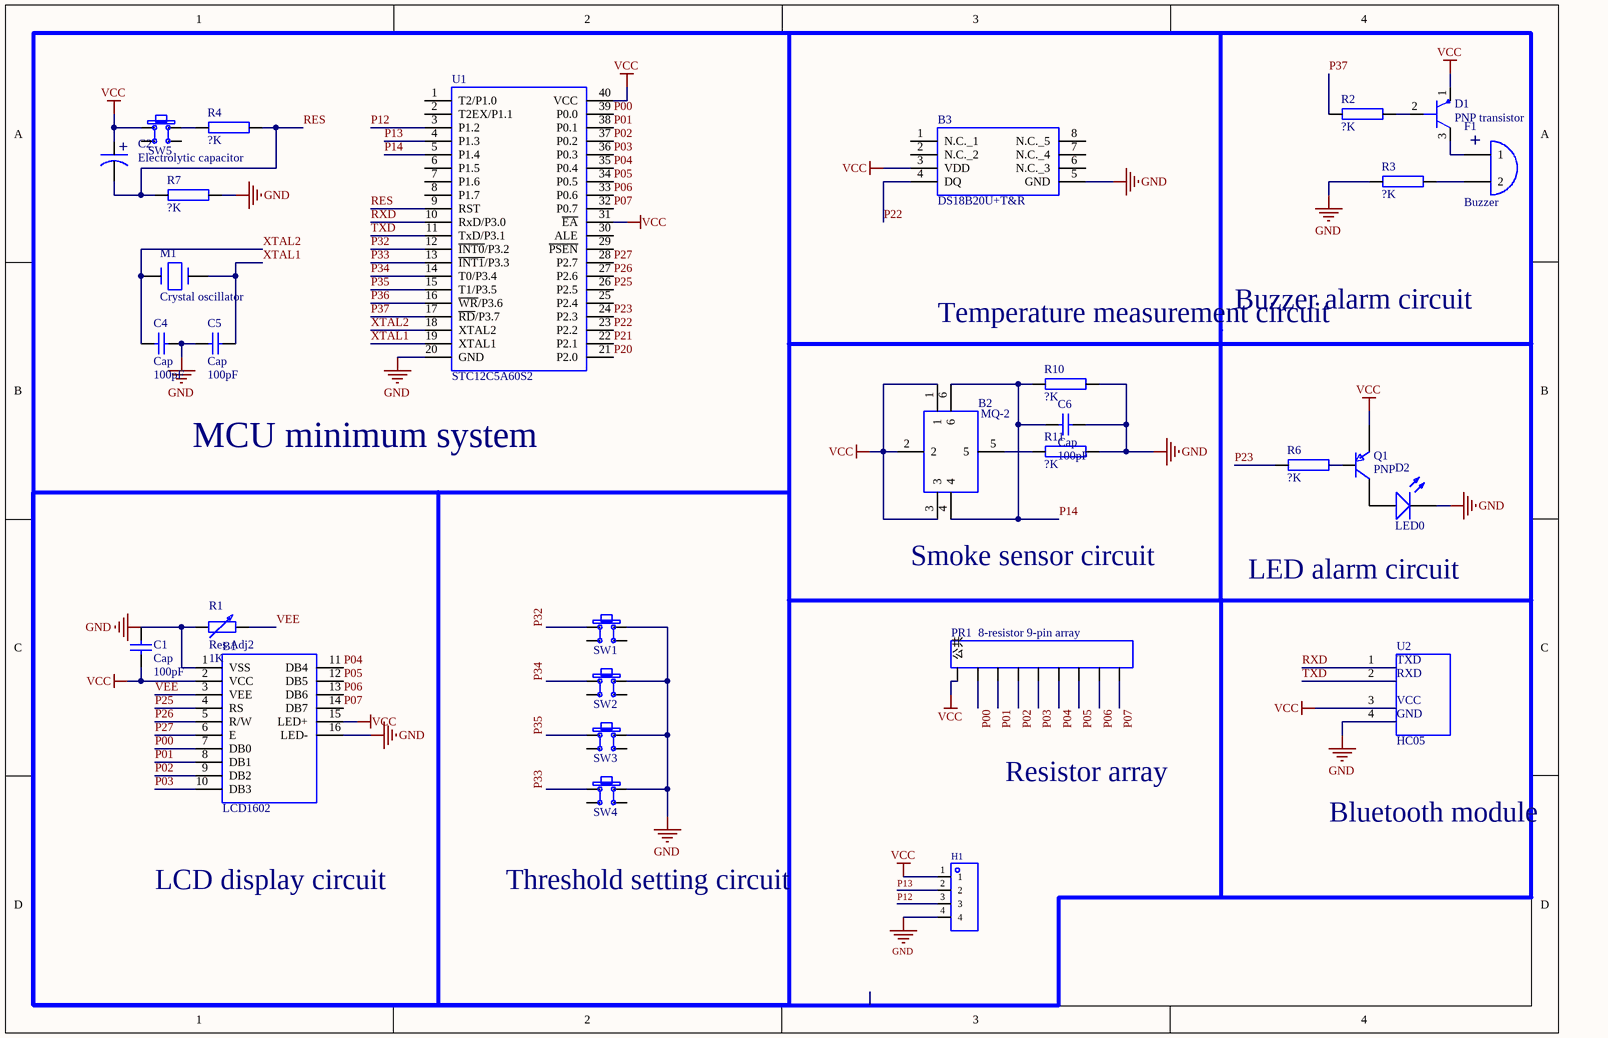
[diagram p0: MISC75421-3.schdoc]
# Altium project MISC75421-2.PrjPcb
1 sheet, 30 parts. Net scope: global (net labels, ports and power ports of the same name join across sheets).
Board file: MISC75421.pcbdoc

## Sheet MISC75421-3.schdoc
size 292 x 193 mm; Name: MISC75421

### Parts
B1  LCD1602  [LCD1602]
B2  MQ-2  [SENSOR-TH_MQ-2]
B3  DS18B20U+T&R  [HDR-TH_8P-P2.54-V-F-R2-C4-S2.54-1]
C1  Cap  value 100pF  [RAD-0.3]
C2  Electrolytic capacitor  [CAP-TH_BD5.0-P2.00-D0.8-FD-10UF50VC110GL]
C4  Cap  value 100pF  [RAD-0.3]
C5  Cap  value 100pF  [RAD-0.3]
C6  Cap  value 100pF  [RAD-0.3]
D1  PNP transistor  [S8550P_TO-92]
D2  LED0  [LED-TH_5mm]
F1  Buzzer  [BUZ-TH_BD12.0-P6.00-D0.9-RD]
H1  (no value)  [HDR-TH_4P-P2.54-V-F]
M1  Crystal oscillator  [HC-49S_L11.5-W5.0-P4.88]
PR1  8-resistor 9-pin array  [RES-ARRAY-TH_9P-P2.54-D1.0]
Q1  PNP  [TO-92-3_L4.6-W3.6-P1.27-L_1]
R1  Res Adj2  value 1K  [RES-ADJ-TH_3P-L9.5-W4.85-P2.54_PV36W103C01B00]
R2  ?K  [Res_1/4W]
R3  ?K  [Res_1/4W]
R4  ?K  [Res_1/4W]
R6  ?K  [Res_1/4W]
R7  ?K  [Res_1/4W]
R10  ?K  [Res_1/4W]
R11  ?K  [Res_1/4W]
SW1  TSW tactile switch  [SW-TH_4P-L6.0-W6.0-P4.50-LS6.5]  (value not drawn)
SW2  TSW tactile switch  [SW-TH_4P-L6.0-W6.0-P4.50-LS6.5]  (value not drawn)
SW3  TSW tactile switch  [SW-TH_4P-L6.0-W6.0-P4.50-LS6.5]  (value not drawn)
SW4  TSW tactile switch  [SW-TH_4P-L6.0-W6.0-P4.50-LS6.5]  (value not drawn)
SW5  TSW tactile switch  [SW-TH_4P-L6.0-W6.0-P4.50-LS6.5]  (value not drawn)
U1  STC12C5A60S2  [DIP-40_L52.3-W13.9-P2.54-LS15.2-BL-BASE]
U2  HC05  [HDR-TH_4P-P2.54-V-F]

### Nets
GND: B1.1(VSS) B1.16(LED-) B3.5(GND) C1.2 C4.2 C5.1 C6.1 D2.2(K) H1.4 R1.1 R3.2 R7.2 R10.2 R11.2 SW1.4 SW2.4 SW3.4 SW4.4 U1.20(GND) U2.4(GND)
VCC: B1.2(VCC) B1.15(LED+) B2.1 B2.2 B2.3 B3.3(VDD) C1.1 C2.1 D1.1(E) H1.1 PR1.1(公共) Q1.3(E) SW5.1 U1.31(~{EA}) U1.40(VCC) U2.3(VCC)
P00: B1.7(DB0) PR1.2 U1.39(P0.0)
P01: B1.8(DB1) PR1.3 U1.38(P0.1)
P02: B1.9(DB2) PR1.4 U1.37(P0.2)
P03: B1.10(DB3) PR1.5 U1.36(P0.3)
P04: B1.11(DB4) PR1.6 U1.35(P0.4)
P05: B1.12(DB5) PR1.7 U1.34(P0.5)
P06: B1.13(DB6) PR1.8 U1.33(P0.6)
P07: B1.14(DB7) PR1.9 U1.32(P0.7)
P12: H1.3 U1.3(P1.2)
P13: H1.2 U1.4(P1.3)
P14: B2.4 B2.6 C6.2 R10.1 U1.5(P1.4)
P20: U1.21(P2.0)
P21: U1.22(P2.1)
P22: B3.4(DQ) U1.23(P2.2)
P23: R6.1 U1.24(P2.3)
P25: B1.4(RS) U1.26(P2.5)
P26: B1.5(R/W) U1.27(P2.6)
P27: B1.6(E) U1.28(P2.7)
P32: SW1.1 U1.12(~{INT0}/P3.2)
P33: SW4.1 U1.13(~{INT1}/P3.3)
P34: SW2.1 U1.14(T0/P3.4)
P35: SW3.1 U1.15(T1/P3.5)
P36: U1.16(~{WR}/P3.6)
P37: R2.1 U1.17(~{RD}/P3.7)
RES: C2.2 R4.2 R7.1 U1.9(RST)
RXD: U1.10(RxD/P3.0) U2.1(TXD)
TXD: U1.11(TxD/P3.1) U2.2(RXD)
VEE: B1.3(VEE) R1.2
XTAL1: C5.2 M1.2 U1.19(XTAL1)
XTAL2: C4.1 M1.1 U1.18(XTAL2)
NetB2_5: B2.5 R11.1
NetD1_2: D1.2(B) R2.2
NetD1_3: D1.3(C) F1.1
NetD2_1: D2.1(A) Q1.1(C)
NetF1_2: F1.2 R3.1
NetQ1_2: Q1.2(B) R6.2
NetR4_1: R4.1 SW5.4

Not connected (* = marked no-connect by the designer): B3 1(N.C._1) 2(N.C._2) 6(N.C._3) 7(N.C._4) 8(N.C._5); SW1 2 3; SW2 2 3; SW3 2 3; SW4 2 3; SW5 2 3; U1 1(T2/P1.0) 2(T2EX/P1.1) 6(P1.5) 7(P1.6) 8(P1.7) 25(P2.4) 29(~{PSEN}) 30(ALE)

### Notes on the sheet
- Buzzer alarm circuit
- Temperature measurement circuit
- MCU minimum system
- (near B2) Smoke sensor circuit
- LED alarm circuit
- Resistor array
- Bluetooth module
- LCD display circuit
- Threshold setting circuit

### Library data of the parts
B1 = LCD1602: Character LCD Module 1602 Built in Controller St7066u COB Type LCD; Manufacturer_Name: Waveshare; Geometry.Height: 14mm; UniqueId: ecd4cc2f475f8764; AddInBom: yes; ModelId: f9d832f46a914cadb50fc4d4cefd2517; Device: LCD1602; Manufacturer_Part_Number: LCD1602; Mouser Part Number: *; Mouser Price/Stock: *; Arrow Part Number: *; Arrow Price/Stock: *; Datasheet Link: https://www.waveshare.com/datasheet/LCD_en_PDF/LCD1602.pdf; DesignItemID: LCD1602; LibraryName: LCD1602; SymbolName: LCD1602; FootprintName: LCD1602; ModelName: LCD1602; ConvertToPcb: yes
B2 = MQ-2: Sensor: gas; smoke,combustible gases; Range: 30010000ppm; MQ-2; Manufacturer_Name: WINSEN; Geometry.Height: 15mm; Origin Footprint: MQ2; UniqueId: 09c8abc5601f23af; AddInBom: yes; Device: MQ-2; Manufacturer_Part_Number: MQ-2; Mouser Part Number: *; Mouser Price/Stock: *; Arrow Part Number: *; Arrow Price/Stock: *; Datasheet Link: https://www.tme.com/Document/9f6250807cbcd9cc73a92775a9c66d2e/MQ-2.pdf; DesignItemID: MQ-2; LibraryName: MQ-2; SymbolName: MQ-2
B3 = DS18B20U+T&R: Board Mount Temperature Sensors Prgmble Resolution 1-Wire Parasite Pwr; Manufacturer_Name: Analog Devices; Geometry.Height: 1.1mm; Origin Footprint: SOP65P490X110-8N; UniqueId: 602cac6f5ce6261d; AddInBom: yes; Device: DS18B20U+T&R; Manufacturer_Part_Number: DS18B20U+T&R; Mouser Part Number: 700-DS18B20UT&R; Mouser Price/Stock: https://www.mouser.co.uk/ProductDetail/Analog-Devices-Maxim-Integrated/DS18B20U%2bTR?qs=7H2Jq%252ByxpJI1ACKb6RIQLA%3D%3D; Arrow Part Number: DS18B20U+T&R; Arrow Price/Stock: https://www.arrow.com/en/products/ds18b20utr/analog-devices?utm_currency=USD&region=nac; Datasheet Link: https://datasheets.maximintegrated.com/en/ds/DS18B20.pdf; DesignItemID: DS18B20U+T&R; LibraryName: DS18B20U+T&R; SymbolName: DS18B20U+T&R
C1 = Cap: Capacitor; UniqueId: 5fb4f22ffcb6a001; AddInBom: yes; Device: Cap; Published: 8-Jun-2000; LatestRevisionDate: 17-Jul-2002; LatestRevisionNote: Re-released for DXP Platform.; PackageReference: RAD-0.3; PackageDescription: Radial Cap, Thru-Hole; 2 Leads; 0.3 in Pin Spacing; DesignItemID: Cap; LibraryName: Miscellaneous Devices; SymbolName: Cap; FootprintName: RAD-0.3; Publisher: Altium Limited
C2 = 电解电容: Origin Footprint: 电解电容-2.5mm; OriginFootprint 2: 电解电容-5mm; UniqueId: 21d50210554cb61f; AddInBom: yes; Device: Electrolytic capacitor; DesignItemID: 电解电容; LibraryName: Common component library; SymbolName: Electrolytic capacitor
C4 = Cap: Capacitor; UniqueId: 623e2bb2442f04df; AddInBom: yes; Device: Cap; Published: 8-Jun-2000; LatestRevisionDate: 17-Jul-2002; LatestRevisionNote: Re-released for DXP Platform.; PackageReference: RAD-0.3; PackageDescription: Radial Cap, Thru-Hole; 2 Leads; 0.3 in Pin Spacing; DesignItemID: Cap; LibraryName: Miscellaneous Devices; SymbolName: Cap; FootprintName: RAD-0.3; Publisher: Altium Limited
C5 = Cap: Capacitor; UniqueId: 05d417a4d81547fc; AddInBom: yes; Device: Cap; Published: 8-Jun-2000; LatestRevisionDate: 17-Jul-2002; LatestRevisionNote: Re-released for DXP Platform.; PackageReference: RAD-0.3; PackageDescription: Radial Cap, Thru-Hole; 2 Leads; 0.3 in Pin Spacing; DesignItemID: Cap; LibraryName: Miscellaneous Devices; SymbolName: Cap; FootprintName: RAD-0.3; Publisher: Altium Limited
C6 = Cap: Capacitor; UniqueId: d45ffe04e43665a4; AddInBom: yes; Device: Cap; Published: 8-Jun-2000; LatestRevisionDate: 17-Jul-2002; LatestRevisionNote: Re-released for DXP Platform.; PackageReference: RAD-0.3; PackageDescription: Radial Cap, Thru-Hole; 2 Leads; 0.3 in Pin Spacing; DesignItemID: Cap; LibraryName: Miscellaneous Devices; SymbolName: Cap; FootprintName: RAD-0.3; Publisher: Altium Limited
D1 = PNP三极管: UniqueId: 07a0d5848cd81316; AddInBom: yes; Device: PNP transistor; Origin Footprint: Transistor; DesignItemID: PNP三极管; LibraryName: Dedicated component library; SymbolName: PNP transistor; ConvertToPcb: yes
D2 = LED0: Typical INFRARED GaAs LED; Origin Footprint: LED-0; UniqueId: fa5cd661465da5bc; AddInBom: yes; Device: LED0; Published: 8-Jun-2000; LatestRevisionDate: 08-Jul-2005; LatestRevisionNote: Mech Layer 1 removed.; PackageReference: LED-0; PackageDescription: LED; 2 Leads; DesignItemID: LED0; LibraryName: Miscellaneous Devices; SymbolName: LED0; Publisher: Altium Limited
F1 = 蜂鸣器: UniqueId: 0327748d3d32b991; AddInBom: yes; Device: Buzzer; Origin Footprint: Buzzer; DesignItemID: 蜂鸣器; LibraryName: Dedicated component library; SymbolName: Buzzer
H1 = HDR-F_2.54_1x4P: Symbol: 2.54-1*4P female; ConvertToPcb: yes; ModelId: d187812051054f85879fcaa51a310d8e0819f05c4eef4c71ace90d822a990e87; ModelTransform: 419.6842,98.464,0,0,0,0,0,0,-118.11; Device: HDR-F_2.54_1x4P; AddInBom: yes; SupplierPart: C2718488; Supplier Footprint: 插件; FootprintName: HDR-TH_4P-P2.54-V-F; ModelName: HDR-TH_4P-P2.54-V-F
M1 = 晶振: UniqueId: dd3285c2b6d2a98e; AddInBom: yes; Device: Crystal oscillator; Origin Footprint: Crystal oscillator; DesignItemID: 晶振; LibraryName: Common component library; SymbolName: Crystal oscillator
PR1 = 8阻9排: UniqueId: d5ea52400f8981b9; AddInBom: yes; Device: 8-resistor 9-pin array; Origin Footprint: 8-resistor 9-pin array; DesignItemID: 8阻9排; LibraryName: Common component library; SymbolName: 8-resistor 9-pin array
Q1 = PNP: PNP Bipolar Transistor; Origin Footprint: SOT-23B_N; OriginFootprint 2: SOT-23B_M; UniqueId: 047b734180970fea; AddInBom: yes; Device: PNP; Published: 8-Jun-2000; LatestRevisionDate: 29-May-2009; LatestRevisionNote: IPC-7351 Footprint Added.; PackageVersion: Aug-1999; PackageReference: SOT-23B; PackageDescription: 3-Pin SOT-23 Package 0.95 mm Pitch, 2.4 mm Lead Span; DesignItemID: PNP; LibraryName: Miscellaneous Devices; SymbolName: PNP; Publisher: Altium Limited
R1 = Res Adj2: Variable Resistor; Set Position: 0.5; Origin Footprint: AXIAL-0.6; UniqueId: 4e166b190d4de1c3; AddInBom: yes; Device: Res Adj2; Published: 8-Jun-2000; LatestRevisionDate: 17-Jul-2002; LatestRevisionNote: Re-released for DXP Platform.; PackageReference: AXIAL-0.6; PackageDescription: Axial Device, Thru-Hole; 2 Leads; 0.6 in Pin Spacing; DesignItemID: Res Adj2; LibraryName: Miscellaneous Devices; SymbolName: Res Adj2; Publisher: Altium Limited
R2 = ？K: Origin Footprint: R general resistor/10mm; UniqueId: 06442d24ab060343; SymbolName: R general resistor; AddInBom: yes; Device: ?K; DesignItemID: R一般电阻; LibraryName: Dedicated component library
R3 = ？K: Origin Footprint: R general resistor/10mm; UniqueId: 6e26aea592918673; SymbolName: R general resistor; AddInBom: yes; Device: ?K; DesignItemID: R一般电阻; LibraryName: Dedicated component library
R4 = ？K: Origin Footprint: R general resistor/10mm; UniqueId: 49359f7360e76581; SymbolName: R general resistor; AddInBom: yes; Device: ?K; DesignItemID: R一般电阻; LibraryName: Dedicated component library
R6 = ？K: Origin Footprint: R general resistor/10mm; UniqueId: c9a24d22ca7022dc; SymbolName: R general resistor; AddInBom: yes; Device: ?K; DesignItemID: R一般电阻; LibraryName: Dedicated component library
R7 = ？K: Origin Footprint: R general resistor/10mm; UniqueId: 01f5c70ff2630ee7; SymbolName: R general resistor; AddInBom: yes; Device: ?K; DesignItemID: R一般电阻; LibraryName: Dedicated component library
R10 = ？K: Origin Footprint: R general resistor/10mm; UniqueId: 7663007c1f2bc029; SymbolName: R general resistor; AddInBom: yes; Device: ?K; DesignItemID: R一般电阻; LibraryName: Dedicated component library
R11 = ？K: Origin Footprint: R general resistor/10mm; UniqueId: 069ba0dc55a84bc8; SymbolName: R general resistor; AddInBom: yes; Device: ?K; DesignItemID: R一般电阻; LibraryName: Dedicated component library
SW1 = TSW 轻触开关: BOM名称: Through-hole 6x6 tactile switch; Origin Footprint: TSW DIP-6*6*5; OriginFootprint 2: TSW DIP-6*6*5_V; OriginFootprint 3: TSW SMD-6*6*5; OriginFootprint 4: TSW SMD-4*4*1.5; OriginFootprint 5: TSW SMD-12*12*5; UniqueId: 1070c7afd779bef2; AddInBom: yes; Device: TSW tactile switch; DesignItemID: TSW 轻触开关; LibraryName: Common component library; Description: TSW tactile switch; SymbolName: TSW tactile switch
SW2 = TSW 轻触开关: BOM名称: Through-hole 6x6 tactile switch; Origin Footprint: TSW DIP-6*6*5; OriginFootprint 2: TSW DIP-6*6*5_V; OriginFootprint 3: TSW SMD-6*6*5; OriginFootprint 4: TSW SMD-4*4*1.5; OriginFootprint 5: TSW SMD-12*12*5; UniqueId: b260d2530c5910ca; AddInBom: yes; Device: TSW tactile switch; DesignItemID: TSW 轻触开关; LibraryName: Common component library; Description: TSW tactile switch; SymbolName: TSW tactile switch
SW3 = TSW 轻触开关: BOM名称: Through-hole 6x6 tactile switch; Origin Footprint: TSW DIP-6*6*5; OriginFootprint 2: TSW DIP-6*6*5_V; OriginFootprint 3: TSW SMD-6*6*5; OriginFootprint 4: TSW SMD-4*4*1.5; OriginFootprint 5: TSW SMD-12*12*5; UniqueId: 7b02e8644b02fe07; AddInBom: yes; Device: TSW tactile switch; DesignItemID: TSW 轻触开关; LibraryName: Common component library; Description: TSW tactile switch; SymbolName: TSW tactile switch
SW4 = TSW 轻触开关: BOM名称: Through-hole 6x6 tactile switch; Origin Footprint: TSW DIP-6*6*5; OriginFootprint 2: TSW DIP-6*6*5_V; OriginFootprint 3: TSW SMD-6*6*5; OriginFootprint 4: TSW SMD-4*4*1.5; OriginFootprint 5: TSW SMD-12*12*5; UniqueId: 85bf34d54f573a70; AddInBom: yes; Device: TSW tactile switch; DesignItemID: TSW 轻触开关; LibraryName: Common component library; Description: TSW tactile switch; SymbolName: TSW tactile switch
SW5 = TSW 轻触开关: BOM名称: Through-hole 6x6 tactile switch; Origin Footprint: TSW DIP-6*6*5; OriginFootprint 2: TSW DIP-6*6*5_V; OriginFootprint 3: TSW SMD-6*6*5; OriginFootprint 4: TSW SMD-4*4*1.5; OriginFootprint 5: TSW SMD-12*12*5; UniqueId: 7a8616b833d38e72; AddInBom: yes; Device: TSW tactile switch; DesignItemID: TSW 轻触开关; LibraryName: Common component library; Description: TSW tactile switch; SymbolName: TSW tactile switch
U1 = STC12C5A60S2: STC MCU; Origin Footprint: DIP40-600; UniqueId: 48a4a086d8c42a18; SymbolName: STC89C52RC; AddInBom: yes; Device: STC12C5A60S2; BOM名称: STC MCU; DesignItemID: STC89C52RC; LibraryName: 3.3 - STC series MCU
U2 = HC05: UniqueId: d74c11912b695046; AddInBom: yes; Device: HC05; DesignItemID: HC05; LibraryName: HC_05; SymbolName: HC05